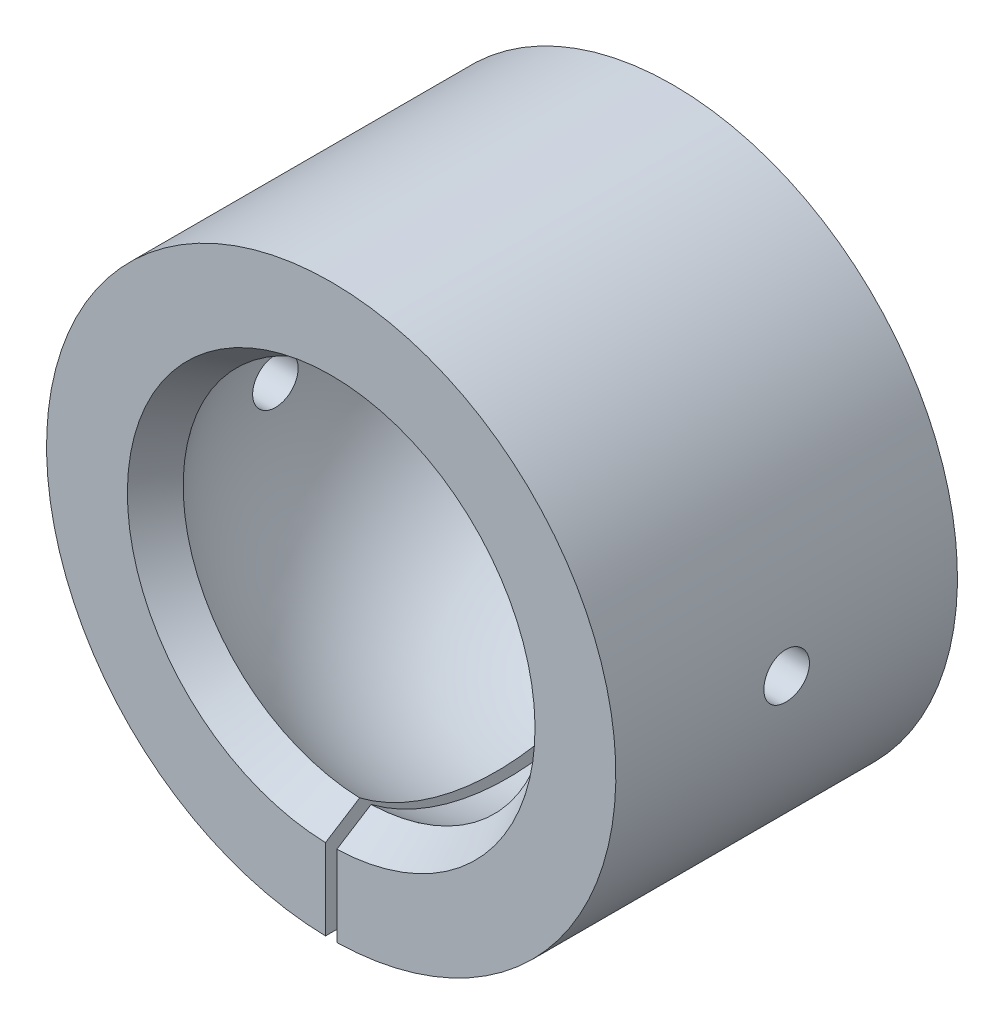
SolidWorks part; units mm, degrees
material "1.7035 (41Cr4)"
ref_plane "前视基准面" through (0, 0, 0) normal (0, 0, 1) x (1, 0, 0)
ref_plane "上视基准面" through (0, 0, 0) normal (0, 1, 0) x (1, 0, 0)
ref_plane "右视基准面" through (0, 0, 0) normal (1, 0, 0) x (0, 0, -1)
sketch "草图1" plane through (0, 0, 0) normal (0, 1, 0) x (1, 0, 0)
  line L0 (0, 23.6294) -> (0, -25.9558) construction
  line L1 (-25.3289, 0) -> (19.5175, 0) construction
  line L2 (17.9, -15) -> (16, -12)
  line L3 (13.2288, 15) -> (25, 15)
  line L5 (17.9, -15) -> (25, -15)
  line L6 (25, 15) -> (25, -15)
  arc A1 (16, -12) -> (13.2288, 15) centre (0, 0) ccw
  dimension "D3" = 20
  dimension "D1" = 50
  dimension "D2" = 30
  dimension "D4" = 32
  dimension "D5" = 35.8
revolve "旋转1" add sketch "草图1" angle 360 about L0
sketch "草图2" plane through (0, 0, 0) normal (0, 1, 0) x (1, 0, 0)
  line L0 (-42.0549, 0) -> (39.4178, 0) construction
  line L1 (0, 42.9571) -> (0, -41.708) construction
  line L5 (-0.5, 17.5) -> (0.5, 17.5)
  line L6 (-0.5, 17.5) -> (-0.5, -17.5)
  line L7 (-0.5, -17.5) -> (0.5, -17.5)
  line L8 (0.5, 17.5) -> (0.5, -17.5)
  dimension "D1" = 35
  dimension "D2" = 1
extrude "切除-拉伸1" cut sketch "草图2" against normal through all
sketch "草图3" plane through (0, 0, 0) normal (1, 0, 0) x (0, 0, -1)
  circle A0 centre (0, 0) radius 2
  dimension "D1" = 4
extrude "切除-拉伸2" cut sketch "草图3" against normal through all both and the other way through all
